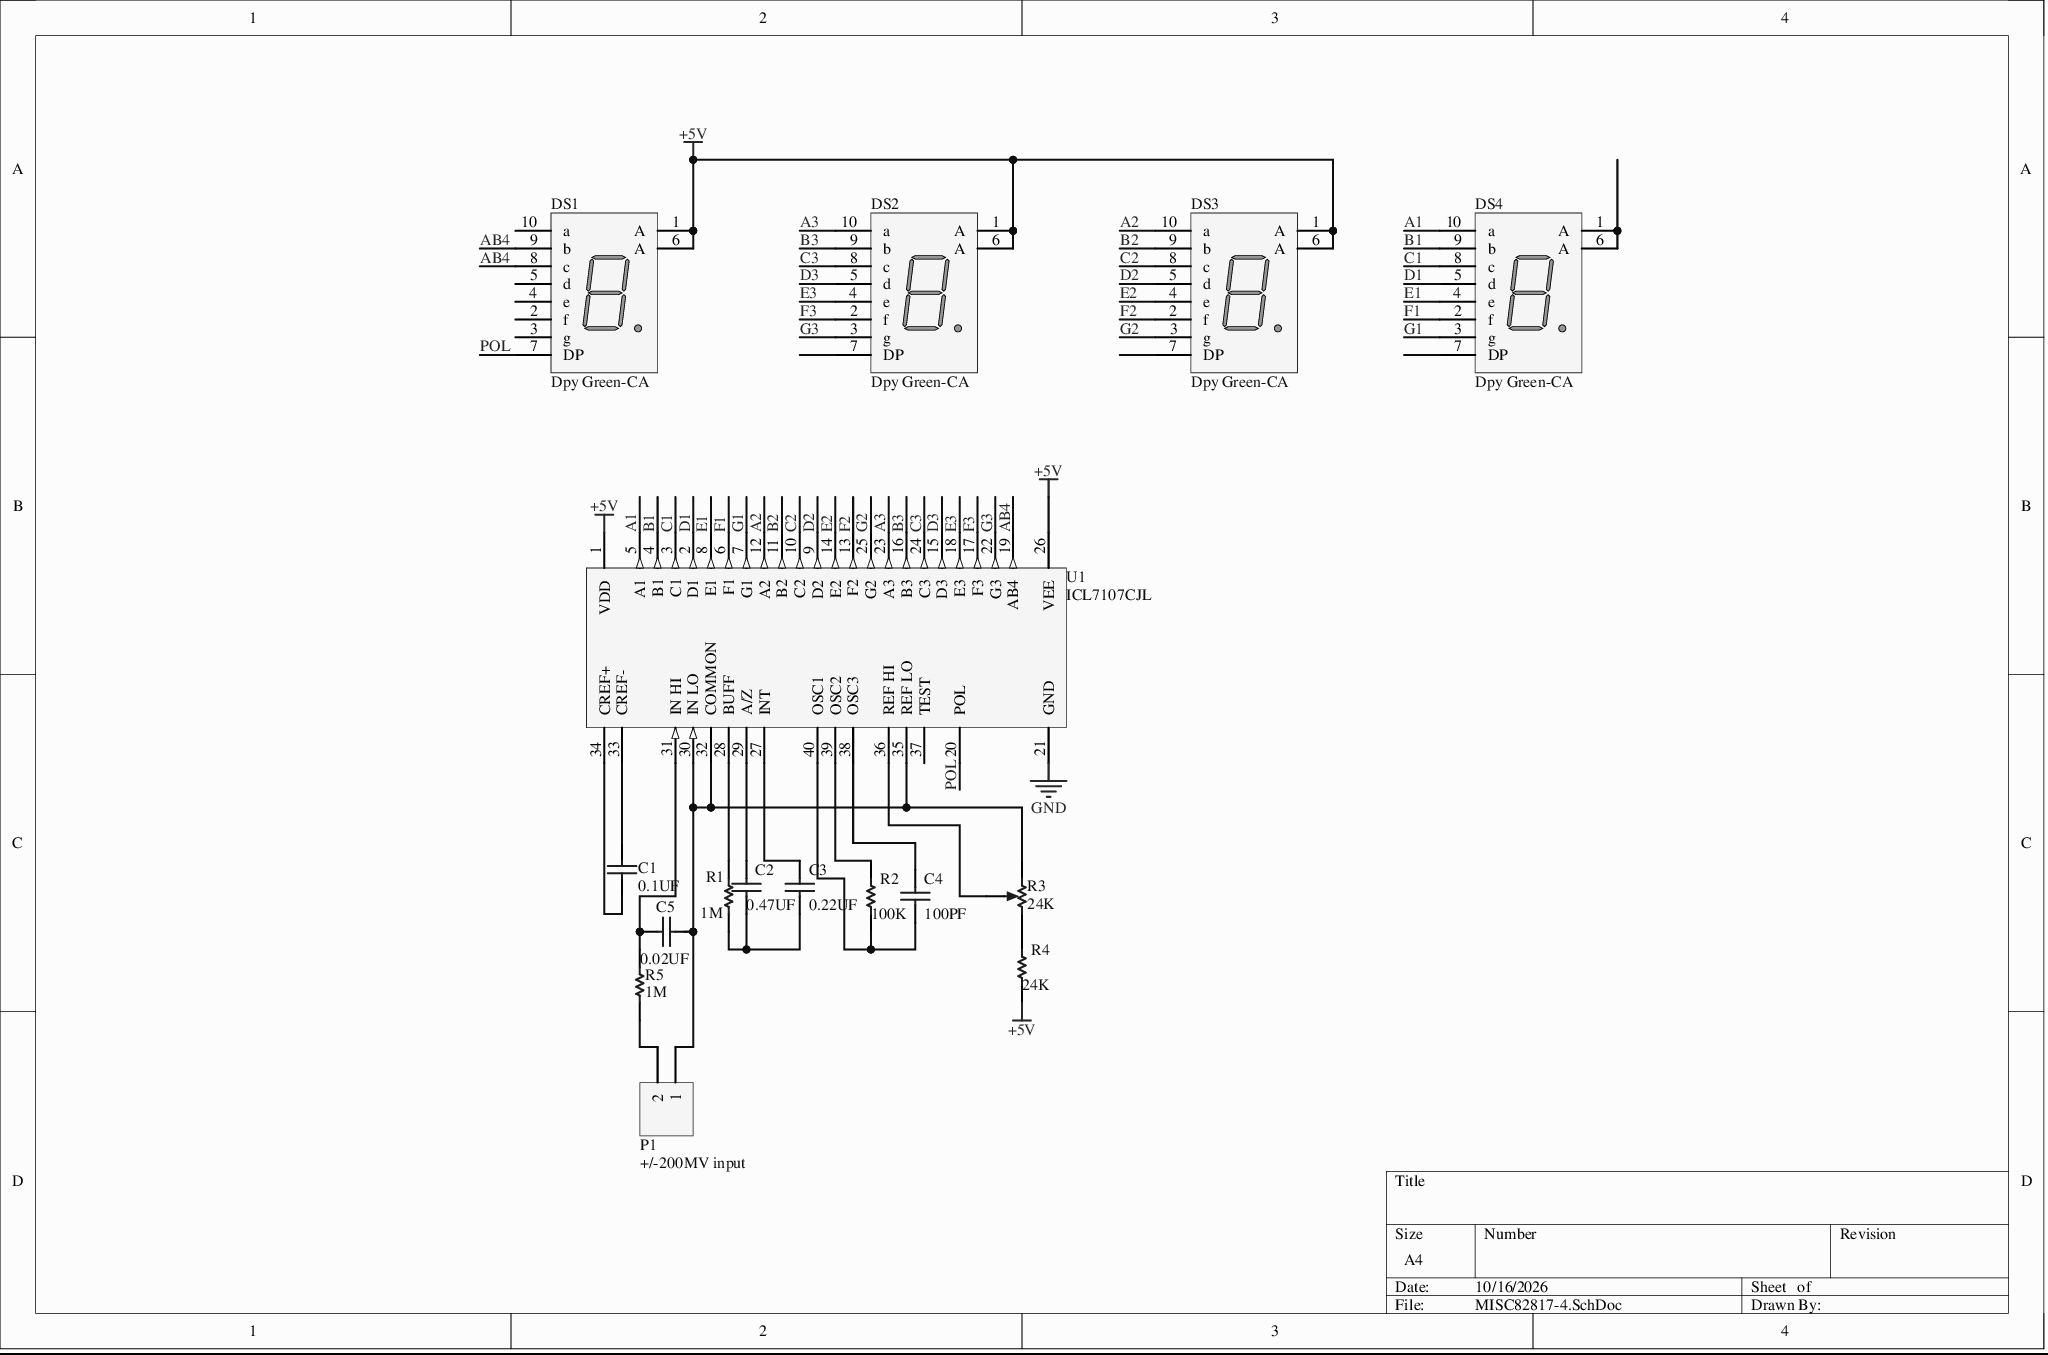
[diagram p0: MISC82817-4.SchDoc]
# Altium project MISC82817-7.PrjPcb
1 sheet, 16 parts. Net scope: global (net labels, ports and power ports of the same name join across sheets).
Board file: MISC82817.PcbDoc

## Sheet MISC82817-4.SchDoc
size A4

### Parts
C1  0.1UF  [RAD-0.3]
C2  0.47UF  [RAD-0.3]
C3  0.22UF  [RAD-0.3]
C4  100PF  [RAD-0.3]
C5  0.02UF  [RAD-0.3]
DS1  Dpy Green-CA  [A]
DS2  Dpy Green-CA  [A]
DS3  Dpy Green-CA  [A]
DS4  Dpy Green-CA  [A]
P1  +/-200MV input  [HDR1X2]
R1  1M  [AXIAL-0.3]
R2  100K  [AXIAL-0.3]
R3  24K  [VR5]
R4  24K  [AXIAL-0.3]
R5  1M  [AXIAL-0.3]
U1  ICL7107CJL  [JL40A]

### Nets
+5V: DS1.1(A) DS1.6(A) DS2.1(A) DS2.6(A) DS3.1(A) DS3.6(A) R4.1 U1.1(VDD) U1.26(VEE)
GND: U1.21(GND)
A1: DS4.10(a) U1.5(A1)
A2: DS3.10(a) U1.12(A2)
A3: DS2.10(a) U1.23(A3)
AB4: DS1.8(c) DS1.9(b) U1.19(AB4)
B1: DS4.9(b) U1.4(B1)
B2: DS3.9(b) U1.11(B2)
B3: DS2.9(b) U1.16(B3)
C1: DS4.8(c) U1.3(C1)
C2: DS3.8(c) U1.10(C2)
C3: DS2.8(c) U1.24(C3)
D1: DS4.5(d) U1.2(D1)
D2: DS3.5(d) U1.9(D2)
D3: DS2.5(d) U1.15(D3)
E1: DS4.4(e) U1.8(E1)
E2: DS3.4(e) U1.14(E2)
E3: DS2.4(e) U1.18(E3)
F1: DS4.2(f) U1.6(F1)
F2: DS3.2(f) U1.13(F2)
F3: DS2.2(f) U1.17(F3)
G1: DS4.3(g) U1.7(G1)
G2: DS3.3(g) U1.25(G2)
G3: DS2.3(g) U1.22(G3)
POL: DS1.7(DP) U1.20(POL)
NetC1_1: C1.1 U1.34(CREF+)
NetC1_2: C1.2 U1.33(CREF-)
NetC2_1: C2.1 U1.29(A/Z)
NetC2_2: C2.2 C3.2 R1.1
NetC3_1: C3.1 U1.27(INT)
NetC4_1: C4.1 U1.38(OSC3)
NetC4_2: C4.2 R2.1 U1.40(OSC1)
NetC5_1: C5.1 P1.1 R3.1(TOP) U1.30(IN_LO) U1.32(COMMON) U1.35(REF_LO)
NetC5_2: C5.2 R5.2 U1.31(IN_HI)
NetDS4_1: DS4.1(A) DS4.6(A)
NetP1_2: P1.2 R5.1
NetR1_2: R1.2 U1.28(BUFF)
NetR2_2: R2.2 U1.39(OSC2)
NetR3_2: R3.2(BOT) R4.2
NetR3_3: R3.3(TAP) U1.36(REF_HI)

Not connected (* = marked no-connect by the designer): DS1 2(f) 3(g) 4(e) 5(d) 10(a); DS2 7(DP); DS3 7(DP); DS4 7(DP); U1 37(TEST)

### Library data of the parts
C1-C3 C5 = Cap: Capacitor; Value: 100pF; Published: 8-Jun-2000; LatestRevisionDate: 17-Jul-2002; LatestRevisionNote: Re-released for DXP Platform.; PackageReference: RAD-0.3; PackageDescription: Radial Cap, Thru-Hole; 2 Leads; 0.3 in Pin Spacing; Publisher: Altium Limited
C4 = Cap: Capacitor; Published: 8-Jun-2000; LatestRevisionDate: 17-Jul-2002; LatestRevisionNote: Re-released for DXP Platform.; PackageReference: RAD-0.3; PackageDescription: Radial Cap, Thru-Hole; 2 Leads; 0.3 in Pin Spacing; Value: 100pF; Publisher: Altium Limited
DS1-DS4 = Dpy Green-CA: 7.62 mm Black Surface Green 7-Segment Display: CA, RH DP; MinimumIntensity: 860 ucd; Note: IF = 10 mA; Note: Pins 1 and 6 are redundant Anodes.; Published: 8-Jun-2000; LatestRevisionDate: 17-Dec-2003; LatestRevisionNote: Schematic revised, PCB Footprint replaced.; DatasheetVersion: 19-Feb-2002; PackageVersion: 11-Feb-2002; PackageReference: A; PackageDescription: LED, 7-Segment Display, 7.62 mm, RHD; 10 Leads; Row Space 5.08 mm; Pitch 2.54 mm; Colour: Green; ComponentLink1Description: Manufacturer Link; Publisher: Altium Limited
P1 = Header 2: Header, 2-Pin; LatestRevisionDate: 17-Jul-2002; LatestRevisionNote: Re-released for DXP Platform.; Publisher: Altium Limited
R1 R2 R4 R5 = Res1: Resistor; Value: 1K; Published: 8-Jun-2000; LatestRevisionDate: 17-Jul-2002; LatestRevisionNote: Re-released for DXP Platform.; PackageReference: AXIAL-0.3; PackageDescription: Axial Device, Thru-Hole; 2 Leads; 0.3 in Pin Spacing; Publisher: Altium Limited
R3 = RPot: Potentiometer; Sim Note: Enter the Resistance value and the set point into parameter fields.; Set Position: 0.5; Value: 1K; Published: 8-Jun-2000; LatestRevisionDate: 17-Jul-2002; LatestRevisionNote: Re-released for DXP Platform.; PackageReference: VR5; PackageDescription: Variable Resistor, Thru-Hole; 3 Leads; Publisher: Altium Limited
U1 = ICL7107CJL: 3?Digit A/D Converter; Code - JEDEC: MS-011-AC; Published: 16-Jan-2001; Revision: 17-Jul-2002: Re-released for DXP Platform.; Datasheet: Latest Revision: 1987; Package Reference: JL40A; Publisher: Altium Limited